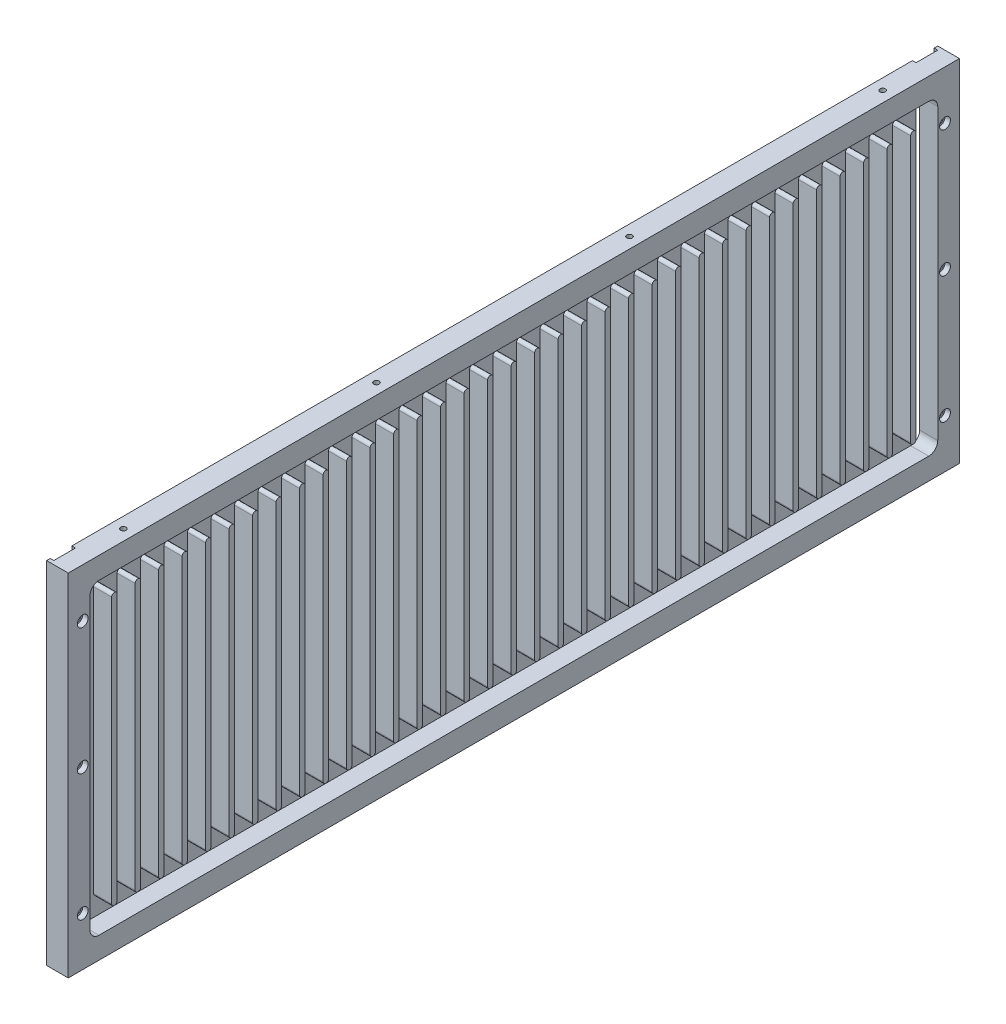
from build123d import *

# Parameters (mm, degrees)
SKETCH1_W           = 493
SKETCH1_H           = 194
BOSS_EXTRUDE1_DEPTH = 6
SKETCH2_W           = 469
SKETCH2_H           = 170
CUT_EXTRUDE1_DEPTH  = 10
BOSS_EXTRUDE2_DEPTH = 10
LPATTERN1_COUNT     = 18
LPATTERN1_PITCH     = 13
LPATTERN1_COL_COUNT = 18
LPATTERN1_COL_PITCH = 13
FILLET1_R           = 5
SKETCH4_R           = 2
CUT_EXTRUDE2_DEPTH  = 266.170228344
SKETCH5_W           = 12
SKETCH5_H           = 194
CUT_EXTRUDE3_DEPTH  = 2
SKETCH6_R           = 1.5
CUT_EXTRUDE4_DEPTH  = 4
SKETCH7_R           = 3
CUT_EXTRUDE5_DEPTH  = 3


with BuildPart() as part:
    # Sketch1 → Boss-Extrude1 (new, symmetric)
    with BuildSketch(Plane(origin=(0, 0, 0), x_dir=(0, 0, -1), z_dir=(1, 0, 0))):
        Rectangle(SKETCH1_W, SKETCH1_H)
    extrude(amount=BOSS_EXTRUDE1_DEPTH, both=True)

    # Sketch2 → Cut-Extrude1 (cut)
    with BuildSketch(Plane(origin=(6, 0, 0), x_dir=(0, 0, -1), z_dir=(1, 0, 0))):
        Rectangle(SKETCH2_W, SKETCH2_H)
    extrude(amount=-CUT_EXTRUDE1_DEPTH, mode=Mode.SUBTRACT)

    # Sketch3 → Boss-Extrude2 (add)
    with BuildSketch(Plane(origin=(-4, 0, 0), x_dir=(0, 0, -1), z_dir=(1, 0, 0))):
        with BuildLine():
            Line((-1.5, 73.5), (-1.5, -73.5))
            ThreePointArc((-1.5, -73.5), (0, -75), (1.5, -73.5))
            Line((1.5, -73.5), (1.5, 73.5))
            ThreePointArc((1.5, 73.5), (0, 75), (-1.5, 73.5))
        make_face()
    boss_extrude2 = extrude(amount=BOSS_EXTRUDE2_DEPTH)

    # LPattern1: Boss-Extrude2 ×18
    with Locations(*[(0, 0, -i * LPATTERN1_PITCH) for i in range(1, LPATTERN1_COUNT)]):
        add(boss_extrude2)

    # LPattern1 col: Boss-Extrude2 ×18
    with Locations(*[(0, 0, i * LPATTERN1_COL_PITCH) for i in range(1, LPATTERN1_COL_COUNT)]):
        add(boss_extrude2)

    # Fillet1
    fillet1_edges = [part.edges().sort_by_distance(p)[0] for p in [
        (1, -85, -234.5),
        (1, -85, 234.5),
        (1, 85, 234.5),
        (1, 85, -234.5),
    ]]
    fillet(fillet1_edges, radius=FILLET1_R)

    # Sketch4 → Cut-Extrude2 (cut, through all)
    with BuildSketch(Plane(origin=(6, 0, 0), x_dir=(0, 0, -1), z_dir=(1, 0, 0))):
        with Locations((-238.5, 0)):
            Circle(SKETCH4_R)
        with Locations((-238.5, 70)):
            Circle(SKETCH4_R)
        with Locations(Location((-238.5, -70, 0), (0, 0, 180))):
            Circle(SKETCH4_R)
    cut_extrude2 = extrude(amount=-CUT_EXTRUDE2_DEPTH, mode=Mode.SUBTRACT)

    # Mirror1: Cut-Extrude2 across plane
    add(cut_extrude2.mirror(Plane.XY), mode=Mode.SUBTRACT)

    # Sketch5 → Cut-Extrude3 (cut)
    with BuildSketch(Plane.ZY.offset(6)):
        with Locations((238.5, 0)):
            Rectangle(SKETCH5_W, SKETCH5_H)
    cut_extrude3 = extrude(amount=-CUT_EXTRUDE3_DEPTH, mode=Mode.SUBTRACT)

    # Mirror2: Cut-Extrude3 across plane
    add(cut_extrude3.mirror(Plane.XY), mode=Mode.SUBTRACT)

    # Sketch6 → Cut-Extrude4 (cut)
    with BuildSketch(Plane(origin=(0, 97, 0), x_dir=(1, 0, 0), z_dir=(0, 1, 0))):
        with Locations(Location((0, -70, 0), (0, 0, 270))):
            Circle(SKETCH6_R)
        with Locations(Location((0, -210, 0), (0, 0, 270))):
            Circle(SKETCH6_R)
        with Locations(Location((0, 210, 0), (0, 0, 90))):
            Circle(SKETCH6_R)
        with Locations(Location((0, 70, 0), (0, 0, 90))):
            Circle(SKETCH6_R)
    cut_extrude4 = extrude(amount=-CUT_EXTRUDE4_DEPTH, mode=Mode.SUBTRACT)

    # Mirror3: Cut-Extrude4 across plane
    add(cut_extrude4.mirror(Plane.ZX), mode=Mode.SUBTRACT)

    # Sketch7 → Cut-Extrude5 (cut)
    with BuildSketch(Plane(origin=(6, 0, 0), x_dir=(0, 0, -1), z_dir=(1, 0, 0))):
        with Locations((238.5, 0)):
            Circle(SKETCH7_R)
        with Locations((238.5, 70)):
            Circle(SKETCH7_R)
        with Locations((238.5, -70)):
            Circle(SKETCH7_R)
        with Locations((-238.5, -70)):
            Circle(SKETCH7_R)
        with Locations((-238.5, 0)):
            Circle(SKETCH7_R)
        with Locations((-238.5, 70)):
            Circle(SKETCH7_R)
    extrude(amount=-CUT_EXTRUDE5_DEPTH, mode=Mode.SUBTRACT)


solid = part.part
